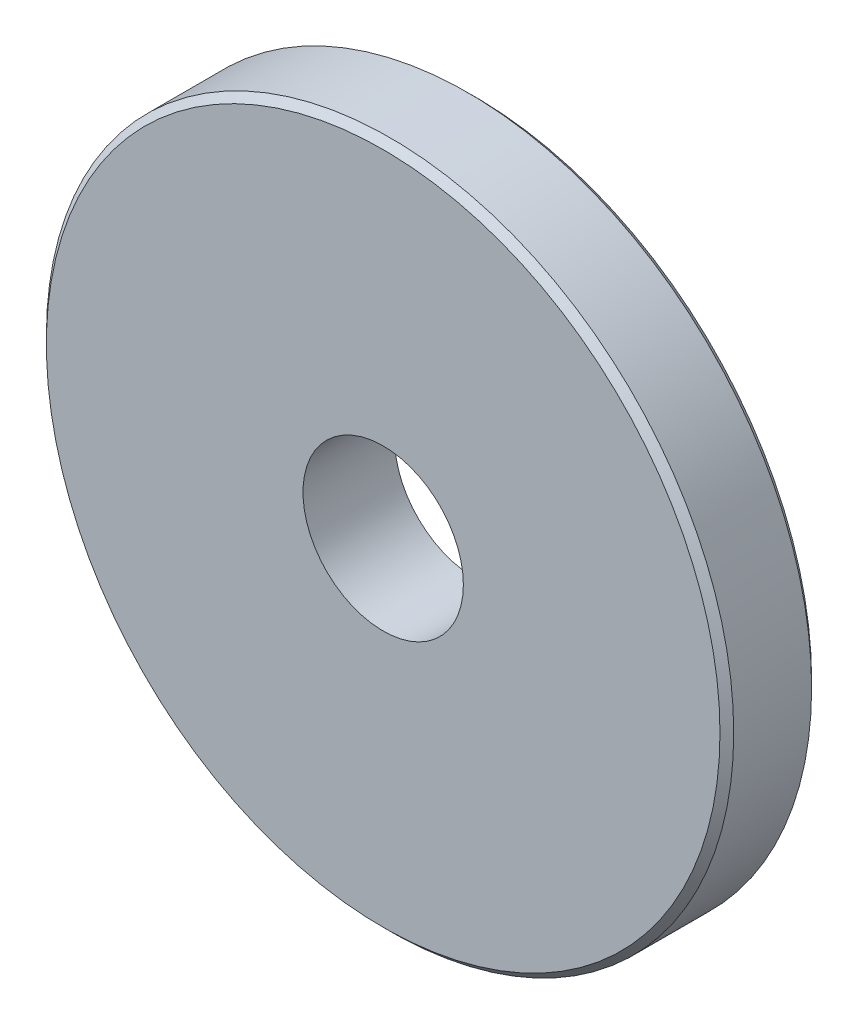
SolidWorks part; units mm, degrees
ref_plane "Front Plane" through (0, 0, 0) normal (0, 0, 1) x (1, 0, 0)
ref_plane "Top Plane" through (0, 0, 0) normal (0, 1, 0) x (1, 0, 0)
ref_plane "Right Plane" through (0, 0, 0) normal (1, 0, 0) x (0, 0, -1)
sketch "Sketch1" plane through (0, 0, 0) normal (0, 0, 1) x (1, 0, 0)
  circle A0 centre (0, 0) radius 15
  circle A1 centre (0, 0) radius 3.5
  dimension "D1" = 30
  dimension "D2" = 7
extrude "Boss-Extrude1" add sketch "Sketch1" along normal blind 4
chamfer "Chamfer1" distance 0.3 angle 45 2 edges at (15, 0, 0) (15, 0, 4)
